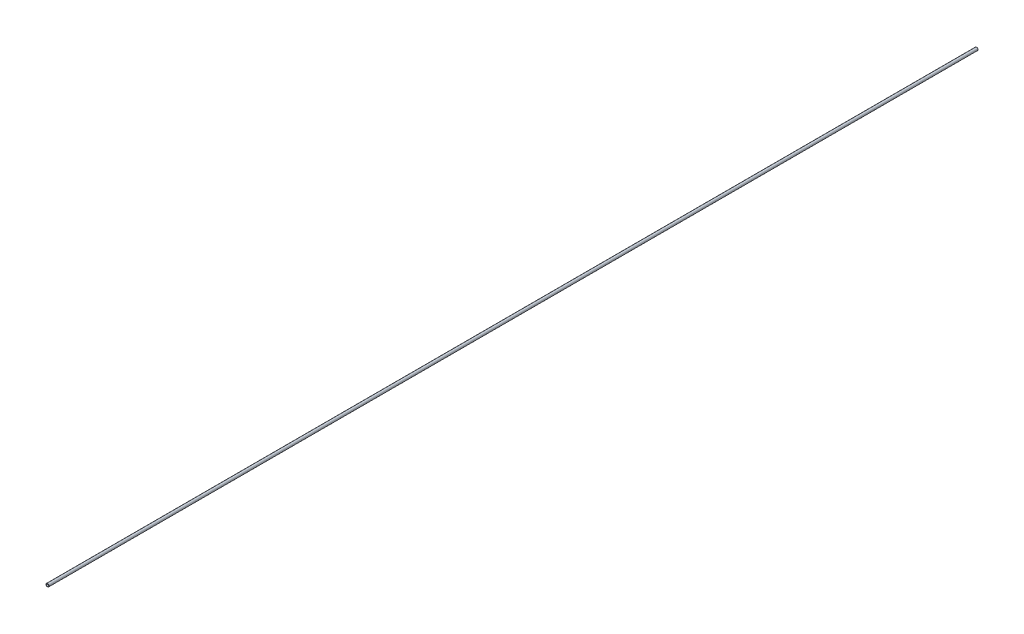
SolidWorks part; units mm, degrees
ref_plane "Front Plane" through (0, 0, 0) normal (0, 0, 1) x (1, 0, 0)
ref_plane "Top Plane" through (0, 0, 0) normal (0, 1, 0) x (1, 0, 0)
ref_plane "Right Plane" through (0, 0, 0) normal (1, 0, 0) x (0, 0, -1)
sketch "Sketch1" plane through (0, 0, 0) normal (0, 0, 1) x (1, 0, 0)
  circle A0 centre (0, 0) radius 2.25
  circle A1 centre (0, 0) radius 3
  dimension "D1" = 6
  dimension "D2" = 4.5
extrude "Boss-Extrude1" add sketch "Sketch1" along normal blind 1900
